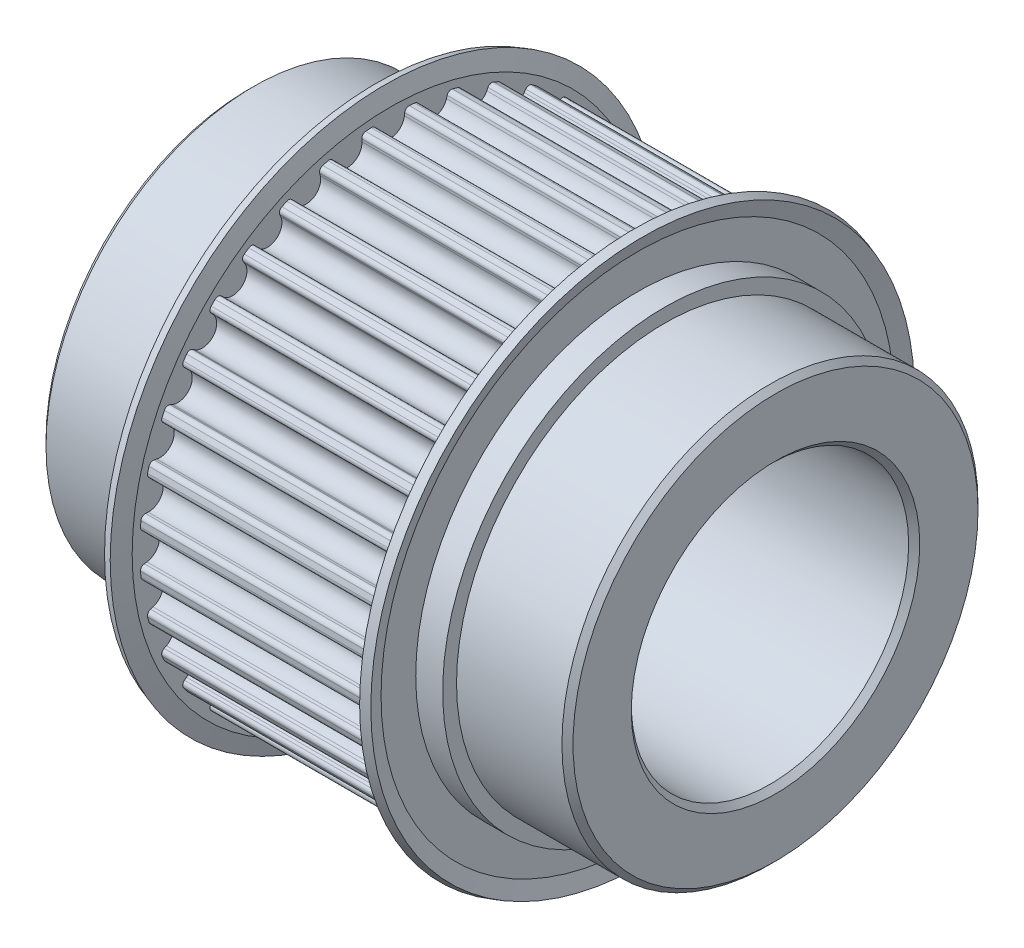
from build123d import *

# Parameters (mm, degrees)
SKETCH1_W           = 48
SKETCH1_H           = 35.6092
CHAMFER1_SIZE       = 1
SKETCH4_W           = 6
SKETCH4_H           = 3.283985022
CUT_EXTRUDE1_DEPTH  = 80.880312981
CUT_EXTRUDE2_REACH  = 81.88
CIRPATTERN3_COUNT   = 36
SKETCH9_OUTSIDE_W   = 119.256
SKETCH9_OUTSIDE_H   = 119.256
SKETCH9_OUTSIDE_R   = 40
CUT_EXTRUDE4_DEPTH  = 2.5
SKETCH7_R           = 40
BOSS_EXTRUDE1_DEPTH = 23.05
CUT_EXTRUDE3_DEPTH  = 65.5
CHAMFER2_SIZE       = 1
SKETCH11_R          = 30
CUT_EXTRUDE5_DEPTH  = 37
SKETCH12_OUTSIDE_W  = 132.4
SKETCH12_OUTSIDE_H  = 132.4
SKETCH12_OUTSIDE_R  = 37.5
CUT_EXTRUDE6_DEPTH  = 20
SKETCH13_R          = 25
CUT_EXTRUDE7_DEPTH  = 71
BOSS_EXTRUDE2_START = 3.95
SKETCH15_R          = 40
SKETCH15_R_2        = 25
BOSS_EXTRUDE2_DEPTH = 3.95
SKETCH16_R          = 37.5
SKETCH16_R_2        = 25
BOSS_EXTRUDE3_DEPTH = 20
CHAMFER3_SIZE       = 1
CHAMFER5_SIZE       = 1


with BuildPart() as part:
    # Sketch1 → Revolve1 (revolve)
    with BuildSketch(Plane.XY, mode=Mode.PRIVATE) as revolve1_sk:
        with Locations((24, 27.3444)):
            Rectangle(SKETCH1_W, SKETCH1_H)
    revolve(revolve1_sk.sketch.rotate(Axis((0, 0, 0), (1, 0, 0)), 90), axis=Axis((0, 0, 0), (1, 0, 0)))

    # Chamfer1
    chamfer1_edges = [part.edges().sort_by_distance(p)[0] for p in [
        (0, 0, -9.5398),
    ]]
    chamfer(chamfer1_edges, length=CHAMFER1_SIZE)

    # Sketch4 → Cut-Extrude1 (cut, through all)
    with BuildSketch(Plane.ZY):
        with Locations((0, 10.697807441)):
            Rectangle(SKETCH4_W, SKETCH4_H)
    extrude(amount=-CUT_EXTRUDE1_DEPTH, mode=Mode.SUBTRACT)

    # Sketch6 → Cut-Extrude2 (cut, up to next)
    with BuildSketch(Plane(origin=(0, 0, 0), x_dir=(0, 0, -1), z_dir=(1, 0, 0)), mode=Mode.PRIVATE) as cut_extrude2_sk1:
        with BuildLine():
            Line((2.608445628, 44.334926581), (2.55084361, 43.865795787))
            ThreePointArc((2.55084361, 43.865795787), (0, 41.609), (-2.55084361, 43.865795787))
            Line((-2.55084361, 43.865795787), (-2.608445628, 44.334926581))
            ThreePointArc((-2.608445628, 44.334926581), (-2.88844915, 44.843344822), (-3.442097755, 45.017598382))
            ThreePointArc((-3.442097755, 45.017598382), (-3.830834279, 44.986185765), (-4.219284955, 44.95141639))
            Line((-4.219284955, 44.95141639), (-4.415932944, 46.552985732))
            ThreePointArc((-4.415932944, 46.552985732), (0, 46.761960442), (4.415932944, 46.552985732))
            Line((4.415932944, 46.552985732), (4.219284955, 44.95141639))
            ThreePointArc((4.219284955, 44.95141639), (3.830834279, 44.986185765), (3.442097755, 45.017598382))
            ThreePointArc((3.442097755, 45.017598382), (2.88844915, 44.843344822), (2.608445628, 44.334926581))
        make_face()
    cut_extrude2_tool1 = extrude(cut_extrude2_sk1.sketch, amount=CUT_EXTRUDE2_REACH, mode=Mode.PRIVATE) & part.part
    cut_extrude2 = cut_extrude2_tool1.solids().sort_by_distance((0, 44.691374, 0))[0]
    add(cut_extrude2, mode=Mode.SUBTRACT)

    # CirPattern3: Cut-Extrude2 ×36 about axis
    cirpattern3_axis = Axis((0, 0, 0), (1, 0, 0))
    for i in range(1, CIRPATTERN3_COUNT):
        add(cut_extrude2.rotate(cirpattern3_axis, i * 360 / CIRPATTERN3_COUNT), mode=Mode.SUBTRACT)

    # Sketch9 outside → Cut-Extrude4 (cut)
    with BuildSketch(Plane(origin=(48, 0, 0), x_dir=(0, 0, -1), z_dir=(1, 0, 0))):
        Rectangle(SKETCH9_OUTSIDE_W, SKETCH9_OUTSIDE_H)
        Circle(SKETCH9_OUTSIDE_R, mode=Mode.SUBTRACT)
    cut_extrude4 = extrude(amount=-CUT_EXTRUDE4_DEPTH, mode=Mode.SUBTRACT)

    # Sketch7 → Boss-Extrude1 (add)
    with BuildSketch(Plane.ZY):
        with Locations(Location((0, 0, 0), (0, 0, 180))):
            Circle(SKETCH7_R)
    extrude(amount=BOSS_EXTRUDE1_DEPTH)

    # Sketch8 → Cut-Extrude3 (cut)
    with BuildSketch(Plane.ZY.offset(23.05)):
        with BuildLine():
            Line((-4, 15.3), (4, 15.3))
            Line((4, 15.3), (4, 11.842719282))
            ThreePointArc((4, 11.842719282), (0, -12.5), (-4, 11.842719282))
            Line((-4, 11.842719282), (-4, 15.3))
        make_face()
    extrude(amount=-CUT_EXTRUDE3_DEPTH, mode=Mode.SUBTRACT)

    # Chamfer2
    chamfer2_edges = [part.edges().sort_by_distance(p)[0] for p in [
        (-23.05, 0, 40),
        (-23.05, -12.5, 0),
    ]]
    chamfer(chamfer2_edges, length=CHAMFER2_SIZE)

    # Mirror1: Cut-Extrude4 across plane
    add(cut_extrude4.mirror(Plane(origin=(24, 0, 0), x_dir=(0, 0, 1), z_dir=(1, 0, 0))), mode=Mode.SUBTRACT)

    # Sketch11 → Cut-Extrude5 (cut)
    with BuildSketch(Plane.ZY.offset(23.05)):
        Circle(SKETCH11_R)
    extrude(amount=-CUT_EXTRUDE5_DEPTH, mode=Mode.SUBTRACT)

    # Sketch12 outside → Cut-Extrude6 (cut)
    with BuildSketch(Plane.ZY.offset(23.05)):
        Rectangle(SKETCH12_OUTSIDE_W, SKETCH12_OUTSIDE_H)
        Circle(SKETCH12_OUTSIDE_R, mode=Mode.SUBTRACT)
    extrude(amount=-CUT_EXTRUDE6_DEPTH, mode=Mode.SUBTRACT)

    # Sketch13 → Cut-Extrude7 (cut)
    with BuildSketch(Plane(origin=(48, 0, 0), x_dir=(0, 0, -1), z_dir=(1, 0, 0))):
        Circle(SKETCH13_R)
    extrude(amount=-CUT_EXTRUDE7_DEPTH, mode=Mode.SUBTRACT)


with BuildPart() as body_2:
    # Sketch10 → Revolve2 (revolve)
    with BuildSketch(Plane.XY, mode=Mode.PRIVATE) as revolve2_sk:
        Polygon((45.5, 40), (45.5, 46.517598382), (46.479952272, 49.5), (48, 49.000545394), (47.097428863, 46.253646695), (47.097428863, 40), align=None)
    revolve(revolve2_sk.sketch.rotate(Axis((0, 0, 0), (1, 0, 0)), 90), axis=Axis((0, 0, 0), (1, 0, 0)))


with BuildPart() as body_3:
    # Mirror2: mirrored copy
    add(body_2.part.mirror(Plane(origin=(24, 0, 0), x_dir=(0, 0, 1), z_dir=(1, 0, 0))))


with BuildPart() as body_2_1:
    add(body_2.part)

    add(part.part)  # Boss-Extrude2 merges part
    # Sketch15 → Boss-Extrude2 (add)
    with BuildSketch(Plane(origin=(48, 0, 0), x_dir=(0, 0, -1), z_dir=(1, 0, 0)).offset(BOSS_EXTRUDE2_START)):
        with Locations(Location((0, 0, 0), (0, 0, 180))):
            Circle(SKETCH15_R)
        Circle(SKETCH15_R_2, mode=Mode.SUBTRACT)
    extrude(amount=-BOSS_EXTRUDE2_DEPTH)

    # Sketch16 → Boss-Extrude3 (add)
    with BuildSketch(Plane(origin=(51.95, 0, 0), x_dir=(0, 0, -1), z_dir=(1, 0, 0))):
        with Locations(Location((0, 0, 0), (0, 0, 180))):
            Circle(SKETCH16_R)
        Circle(SKETCH16_R_2, mode=Mode.SUBTRACT)
    extrude(amount=BOSS_EXTRUDE3_DEPTH)

    # Chamfer3
    chamfer3_edges = [body_2_1.edges().sort_by_distance(p)[0] for p in [
        (-23.05, 0, -37.5),
        (-23.05, 0, -30),
        (71.95, 0, -37.5),
    ]]
    chamfer(chamfer3_edges, length=CHAMFER3_SIZE)

    # Chamfer5
    chamfer5_edges = [body_2_1.edges().sort_by_distance(p)[0] for p in [
        (71.95, 0, 25),
    ]]
    chamfer(chamfer5_edges, length=CHAMFER5_SIZE)


solid = Compound([body_3.part, body_2_1.part])
